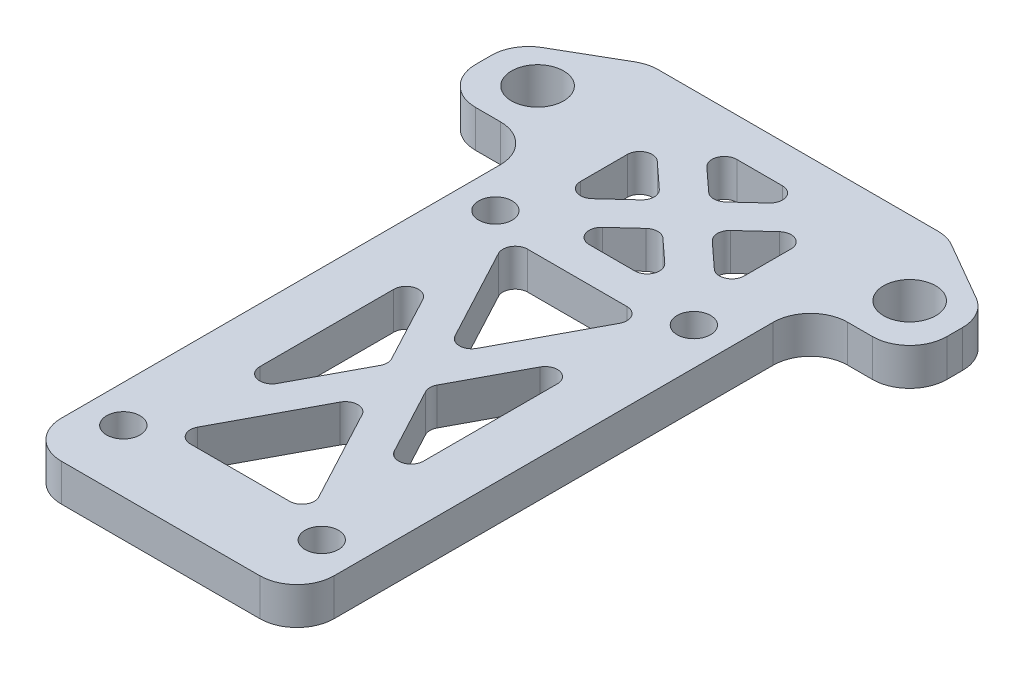
from build123d import *

# Parameters (mm, degrees)
SKETCH1_R              = 2.1
SKETCH1_R_2            = 1.35
BOSS_EXTRUDE1_DEPTH    = 3
CUT_EXTRUDE1_DEPTH     = 50.306794664
R3_OUTER_EDGE_FILLET_R = 3
R1_CUTOUT_FILLET_R     = 1


with BuildPart() as part:
    # Sketch1 → Boss-Extrude1 (new body)
    with BuildSketch(Plane(origin=(0, 0, 0), x_dir=(1, 0, 0), z_dir=(0, 1, 0))):
        Polygon((-12.07179677, 6), (-19, 2), (-19, -4), (-11, -4), (-11, -45.4), (11, -45.4), (11, -4), (19, -4), (19, 2), (12.07179677, 6), align=None)
        with Locations(Location((-15, 0, 0), (0, 0, 270))):
            Circle(SKETCH1_R, mode=Mode.SUBTRACT)
        with Locations(Location((15, 0, 0), (0, 0, 270))):
            Circle(SKETCH1_R, mode=Mode.SUBTRACT)
        with Locations(Location((-8, -10.4, 0), (0, 0, 270))):
            Circle(SKETCH1_R_2, mode=Mode.SUBTRACT)
        with Locations(Location((-8, -40.4, 0), (0, 0, 270))):
            Circle(SKETCH1_R_2, mode=Mode.SUBTRACT)
        with Locations(Location((8, -10.4, 0), (0, 0, 90))):
            Circle(SKETCH1_R_2, mode=Mode.SUBTRACT)
        with Locations(Location((8, -40.4, 0), (0, 0, 90))):
            Circle(SKETCH1_R_2, mode=Mode.SUBTRACT)
    extrude(amount=BOSS_EXTRUDE1_DEPTH)

    # Sketch2 → Cut-Extrude1 (cut, through all)
    with BuildSketch(Plane(origin=(0, 3, 0), x_dir=(1, 0, 0), z_dir=(0, 1, 0))):
        Polygon((-6.6, 1.112582185), (-6.6, -7.212582185), (-2.069298303, -3.05), align=None)
        Polygon((-4.406892174, 2.9), (0, -1.148832185), (4.406892174, 2.9), align=None)
        Polygon((6.6, 1.112582185), (2.069298303, -3.05), (6.6, -7.212582185), align=None)
        Polygon((0, -4.951167815), (-4.406892174, -9), (4.406892174, -9), align=None)
        Polygon((5.666666667, -11.8), (-5.666666667, -11.8), (0, -22.425), align=None)
        Polygon((-1.586666667, -25.4), (-6.6, -16), (-6.6, -34.8), align=None)
        Polygon((5.666666667, -39), (0, -28.375), (-5.666666667, -39), align=None)
        Polygon((6.6, -16), (1.586666667, -25.4), (6.6, -34.8), align=None)
    extrude(amount=-CUT_EXTRUDE1_DEPTH, mode=Mode.SUBTRACT)

    # R3 outer edge fillet
    r3_outer_edge_fillet_edges = [part.edges().sort_by_distance(p)[0] for p in [
        (19, 1.5, 4),
        (11, 1.5, 4),
        (11, 1.5, 45.4),
        (-11, 1.5, 45.4),
        (-11, 1.5, 4),
        (-19, 1.5, 4),
        (-19, 1.5, -2),
        (-12.07179677, 1.5, -6),
        (12.07179677, 1.5, -6),
        (19, 1.5, -2),
    ]]
    fillet(r3_outer_edge_fillet_edges, radius=R3_OUTER_EDGE_FILLET_R)

    # R1 cutout fillet
    r1_cutout_fillet_edges = [part.edges().sort_by_distance(p)[0] for p in [
        (6.6, 1.5, 16),
        (6.6, 1.5, 34.8),
        (1.586666667, 1.5, 25.4),
        (-6.6, 1.5, 34.8),
        (-6.6, 1.5, 16),
        (-1.586666667, 1.5, 25.4),
        (5.666666667, 1.5, 39),
        (-5.666666667, 1.5, 39),
        (0, 1.5, 28.375),
        (-2.069298303, 1.5, 3.05),
        (-6.6, 1.5, 7.212582185),
        (-6.6, 1.5, -1.112582185),
        (-5.666666667, 1.5, 11.8),
        (5.666666667, 1.5, 11.8),
        (0, 1.5, 22.425),
        (0, 1.5, 4.951167815),
        (4.406892174, 1.5, 9),
        (-4.406892174, 1.5, 9),
        (4.406892174, 1.5, -2.9),
        (0, 1.5, 1.148832185),
        (-4.406892174, 1.5, -2.9),
        (6.6, 1.5, -1.112582185),
        (6.6, 1.5, 7.212582185),
        (2.069298303, 1.5, 3.05),
    ]]
    fillet(r1_cutout_fillet_edges, radius=R1_CUTOUT_FILLET_R)


solid = part.part
